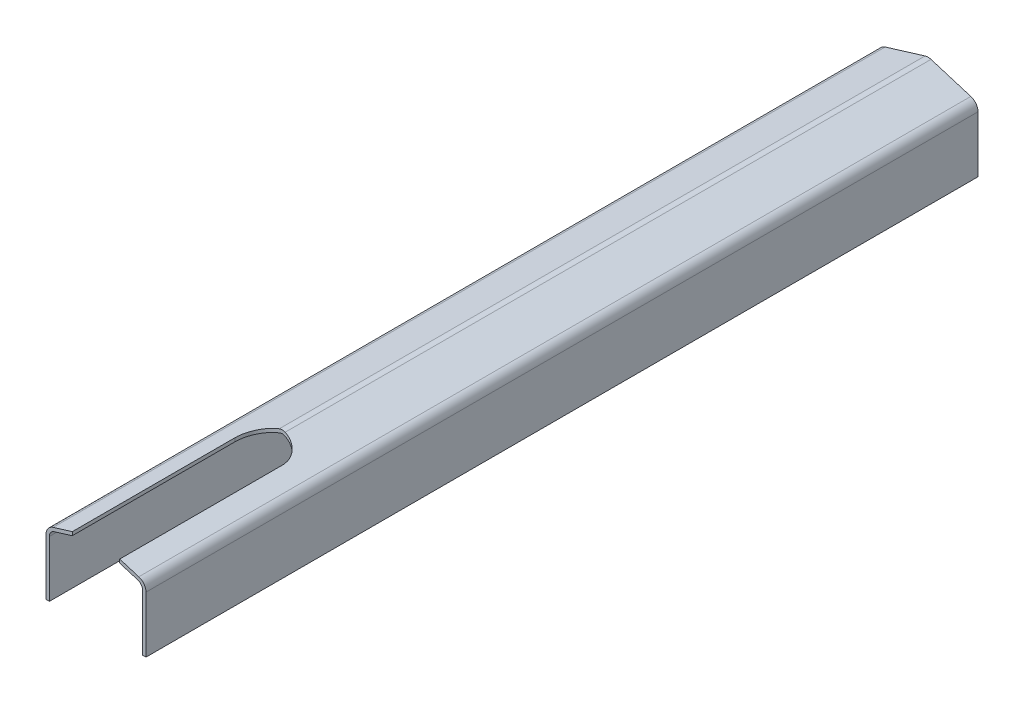
SolidWorks part; units mm, degrees
ref_plane "Front Plane" through (0, 0, 0) normal (0, 0, 1) x (1, 0, 0)
ref_plane "Top Plane" through (0, 0, 0) normal (0, 1, 0) x (1, 0, 0)
ref_plane "Right Plane" through (0, 0, 0) normal (1, 0, 0) x (0, 0, -1)
sketch "Sketch1" plane through (0, 0, 0) normal (0, 0, 1) x (1, 0, 0)
  line L0 (-147.5, 0) -> (-147.5, 166.0766)
  line L1 (-126.2712, 194.7658) -> (-8.7712, 230.6891)
  line L2 (126.2712, 194.7658) -> (8.7712, 230.6891)
  line L3 (147.5, 166.0766) -> (147.5, 0)
  line L4 (137.5, 166.0766) -> (137.5, 0)
  line L5 (0, -24.4365) -> (0, 550.6844) construction
  line L6 (123.3474, 185.2027) -> (5.8474, 221.1261)
  line L7 (-123.3474, 185.2027) -> (-5.8474, 221.1261)
  line L8 (-137.5, 0) -> (-137.5, 166.0766)
  line L9 (-147.5, 0) -> (-137.5, 0)
  line L10 (137.5, 0) -> (147.5, 0)
  arc A0 (8.7712, 230.6891) -> (-8.7712, 230.6891) centre (0, 202) ccw
  arc A1 (147.5, 166.0766) -> (126.2712, 194.7658) centre (117.5, 166.0766) ccw
  arc A2 (-147.5, 166.0766) -> (-126.2712, 194.7658) centre (-117.5, 166.0766) cw
  arc A3 (137.5, 166.0766) -> (123.3474, 185.2027) centre (117.5, 166.0766) ccw
  arc A4 (5.8474, 221.1261) -> (-5.8474, 221.1261) centre (0, 202) ccw
  arc A5 (-137.5, 166.0766) -> (-123.3474, 185.2027) centre (-117.5, 166.0766) cw
  dimension "D3" = 60
  dimension "D7" = 30
  dimension "D1" = 295
  dimension "D2" = 295
  dimension "D4" = 202
  dimension "D5" = 73
  dimension "D6" = 73
  dimension "D8" = 10
extrude "Boss-Extrude1" add sketch "Sketch1" along normal blind 2455
sketch "Sketch2" plane through (0, 0, 0) normal (0, 1, 0) x (1, 0, 0)
  line L0 (0, 0) -> (0, -4105.5152) construction
  line L2 (-70, -1975) -> (-70, -2455)
  line L3 (70, -1975) -> (70, -2455)
  line L4 (-105.6251, -1975) -> (225.2382, -1975) construction
  line L6 (137.5, -2455) -> (147.5, -2455) construction
  line L7 (-70, 0) -> (-70, -4105.5152) construction
  line L8 (70, 0) -> (70, -4105.5152) construction
  line L9 (5.8474, -2455) -> (123.3474, -2455) construction
  line L10 (-70, -2455) -> (70, -2455)
  arc A0 (70, -1975) -> (-70, -1975) centre (0, -1975) ccw
  dimension "D1" = 70
  dimension "D2" = 480
extrude "Cut-Extrude1" cut sketch "Sketch2" along normal through all
sketch "Sketch3" plane through (-147.5, 0, 0) normal (-1, 0, 0) x (0, 0, 1)
  line L2 (1565, 274.6018) -> (1565, -109.9512) construction
  line L3 (2455, 166.0766) -> (2455, 0) construction
  line L4 (2455, 0) -> (0, 0) construction
  line L5 (1545, 137) -> (1585, 137)
  line L6 (1545, 57) -> (1585, 57)
  arc A0 (1545, 137) -> (1545, 57) centre (1545, 97) ccw
  arc A1 (1585, 57) -> (1585, 137) centre (1585, 97) ccw
  dimension "D3" = 80
  dimension "D1" = 40
  dimension "D2" = 80
  dimension "D4" = 890
  dimension "D5" = 20
  dimension "D6" = 97
  dimension "D7" = 97
extrude "Cut-Extrude2" cut sketch "Sketch3" against normal blind 10
hole_wizard "M10 Tapped Hole1" positions "Sketch5" profile "Sketch4" tap size "M10" standard "GB"
sketch "Sketch5" plane through (-147.5, 0, 0) normal (-1, 0, 0) x (0, 0, 1)
  line L3 (1565, 268.0125) -> (1565, -37.5339) construction
  line L4 (2455, 166.0766) -> (2455, 0) construction
  line L5 (1477.9986, 97) -> (1862.7865, 97) construction
  line L6 (2455, 0) -> (0, 0) construction
  point P0 (1565, 147)
  point P1 (1565, 47)
  point P37 (1495, 97)
  point P39 (1635, 97)
  dimension "D1" = 890
  dimension "D2" = 97
  dimension "D3" = 50
  dimension "D4" = 50
  dimension "D5" = 70
  dimension "D6" = 70
sketch "Sketch4" plane through (-147.5, 147, 1565) normal (0, 1, 0) x (0, 0, 1)
  line L0 (0, 0) -> (0, 30.0537)
  line L1 (0, 30.0537) -> (4.25, 27.5)
  line L2 (4.25, 27.5) -> (4.25, 0)
  line L5 (4.25, 0) -> (0, 0)
  line L10 (0, 30.0537) -> (-4.25, 27.5) construction
  line L11 (0, -6.35) -> (0, 107.95) construction
  dimension "螺纹孔钻头直径" = 8.5
  dimension "螺纹孔钻头深度" = 27.5
  dimension "导头角度" = 118
cosmetic thread "Cosmetic Thread 1" parameters "D1"=10, "D2"=10
cosmetic thread "Cosmetic Thread 2" parameters "D1"=10, "D2"=10
cosmetic thread "Cosmetic Thread 3" parameters "D1"=10, "D2"=10
cosmetic thread "Cosmetic Thread 4" parameters "D1"=10, "D2"=10
